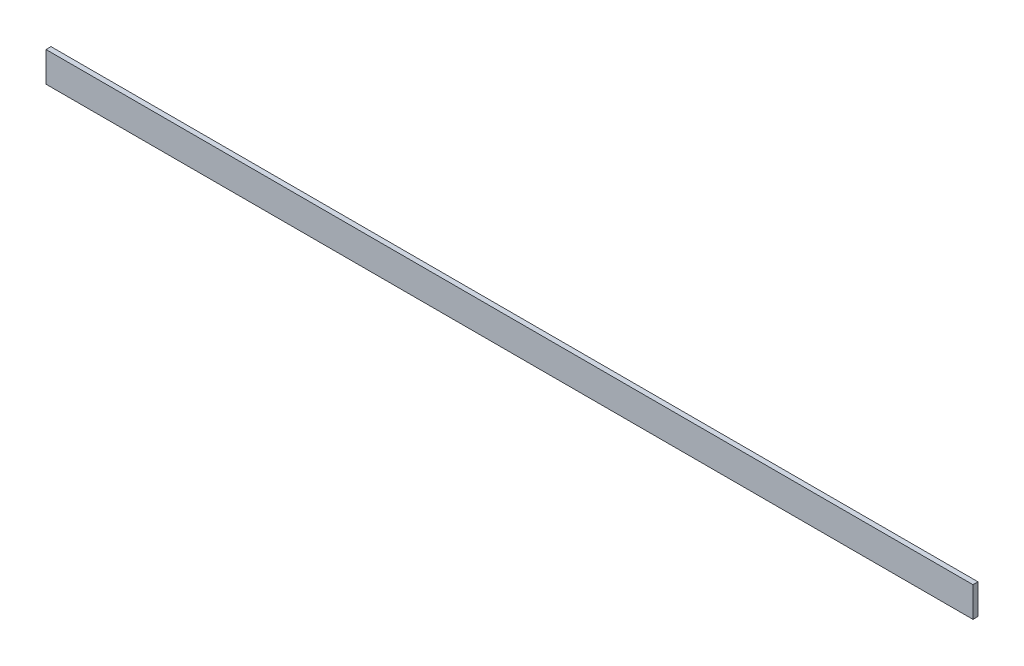
from build123d import *

# Parameters (mm, degrees)
SKETCH1_W           = 925
SKETCH1_H           = 30
BOSS_EXTRUDE1_DEPTH = 5


with BuildPart() as part:
    # Sketch1 → Boss-Extrude1 (new body)
    with BuildSketch(Plane.XY):
        Rectangle(SKETCH1_W, SKETCH1_H)
    extrude(amount=BOSS_EXTRUDE1_DEPTH)


solid = part.part
